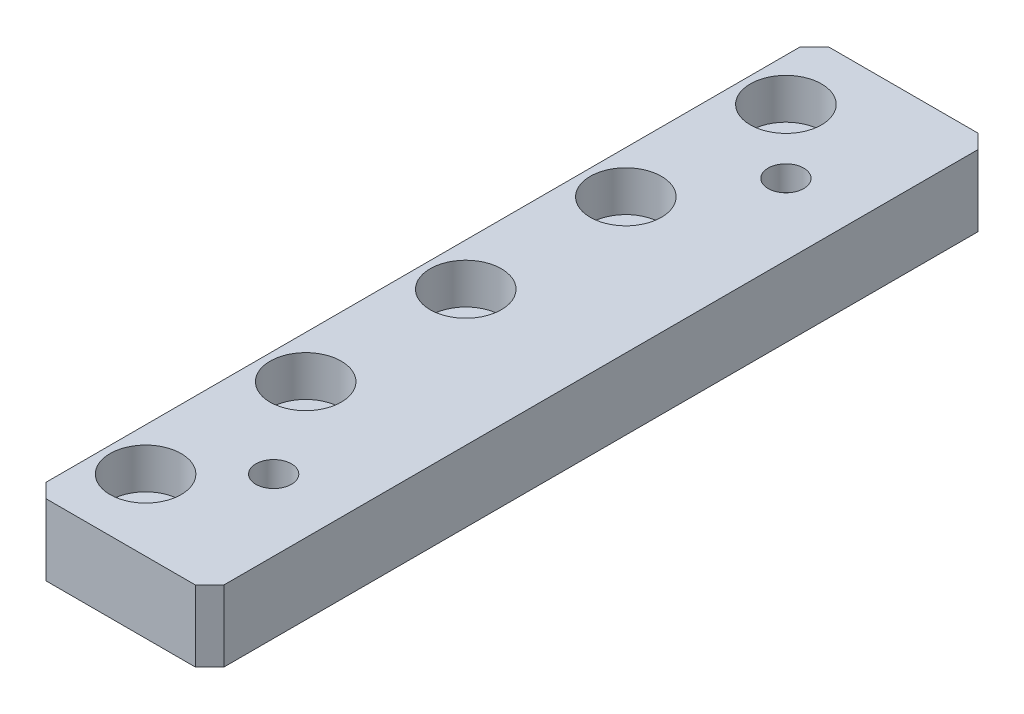
from build123d import *

# Parameters (mm, degrees)
SKETCH_1_W                  = 25
SKETCH_1_H                  = 110
EXTRUDE_1_DEPTH             = 10
CHAMFER_1_SIZE              = 2
HOLE_WIZARD_1_D             = 5.5
HOLE_WIZARD_1_DEPTH         = 12.4
HOLE_WIZARD_1_CBORE_D       = 10
HOLE_WIZARD_1_CBORE_DEPTH   = 5.7
HOLE_WIZARD_1_TIP           = 1.652366702
HOLE_WIZARD_1_2_D           = 3.4
HOLE_WIZARD_1_2_DEPTH       = 15
HOLE_WIZARD_1_2_CBORE_D     = 6
HOLE_WIZARD_1_2_CBORE_DEPTH = 3.4
HOLE_WIZARD_1_2_TIP         = 1.021463052
SKETCH_6_R                  = 2.5
CUT_EXTRUDE_1_DEPTH         = 3.5


with BuildPart() as part:
    # 草图1 → 凸台-拉伸1 (new body)
    with BuildSketch(Plane(origin=(0, 0, 0), x_dir=(1, 0, 0), z_dir=(0, 1, 0))):
        Rectangle(SKETCH_1_W, SKETCH_1_H)
    extrude(amount=EXTRUDE_1_DEPTH)

    # 倒角1
    chamfer_1_edges = [part.edges().sort_by_distance(p)[0] for p in [
        (12.5, 5, 55),
        (-12.5, 5, 55),
        (-12.5, 5, -55),
        (12.5, 5, -55),
    ]]
    chamfer(chamfer_1_edges, length=CHAMFER_1_SIZE)

    # Hole Wizard 1
    with Locations(Plane(origin=(0, 10, 0), x_dir=(1, 0, 0), z_dir=(0, 1, 0))):
        with Locations((-6.5, -45), (-6.5, 0), (-6.5, 45), (-6.5, -22.5), (-6.5, 22.5)):
            CounterBoreHole(HOLE_WIZARD_1_D / 2, HOLE_WIZARD_1_CBORE_D / 2, HOLE_WIZARD_1_CBORE_DEPTH, depth=HOLE_WIZARD_1_DEPTH)
            with Locations((0, 0, -(HOLE_WIZARD_1_DEPTH + HOLE_WIZARD_1_TIP / 2))):  # 118° drill point
                Cone(0, HOLE_WIZARD_1_D / 2, HOLE_WIZARD_1_TIP, mode=Mode.SUBTRACT)

    # Hole Wizard 1 2
    with Locations(Plane(origin=(0, 0, 0), x_dir=(-1, 0, 0), z_dir=(0, -1, 0))):
        with Locations((-2.5, -36), (-2.5, 36)):
            CounterBoreHole(HOLE_WIZARD_1_2_D / 2, HOLE_WIZARD_1_2_CBORE_D / 2, HOLE_WIZARD_1_2_CBORE_DEPTH, depth=HOLE_WIZARD_1_2_DEPTH)
            with Locations((0, 0, -(HOLE_WIZARD_1_2_DEPTH + HOLE_WIZARD_1_2_TIP / 2))):  # 118° drill point
                Cone(0, HOLE_WIZARD_1_2_D / 2, HOLE_WIZARD_1_2_TIP, mode=Mode.SUBTRACT)

    # 草图6 → 切除-拉伸1 (cut)
    with BuildSketch(Plane(origin=(0, 10, 0), x_dir=(1, 0, 0), z_dir=(0, 1, 0))):
        with Locations(Location((2.5, -36, 0), (0, 0, 270))):
            Circle(SKETCH_6_R)
        with Locations(Location((2.5, 36, 0), (0, 0, 270))):
            Circle(SKETCH_6_R)
    extrude(amount=-CUT_EXTRUDE_1_DEPTH, mode=Mode.SUBTRACT)


solid = part.part
